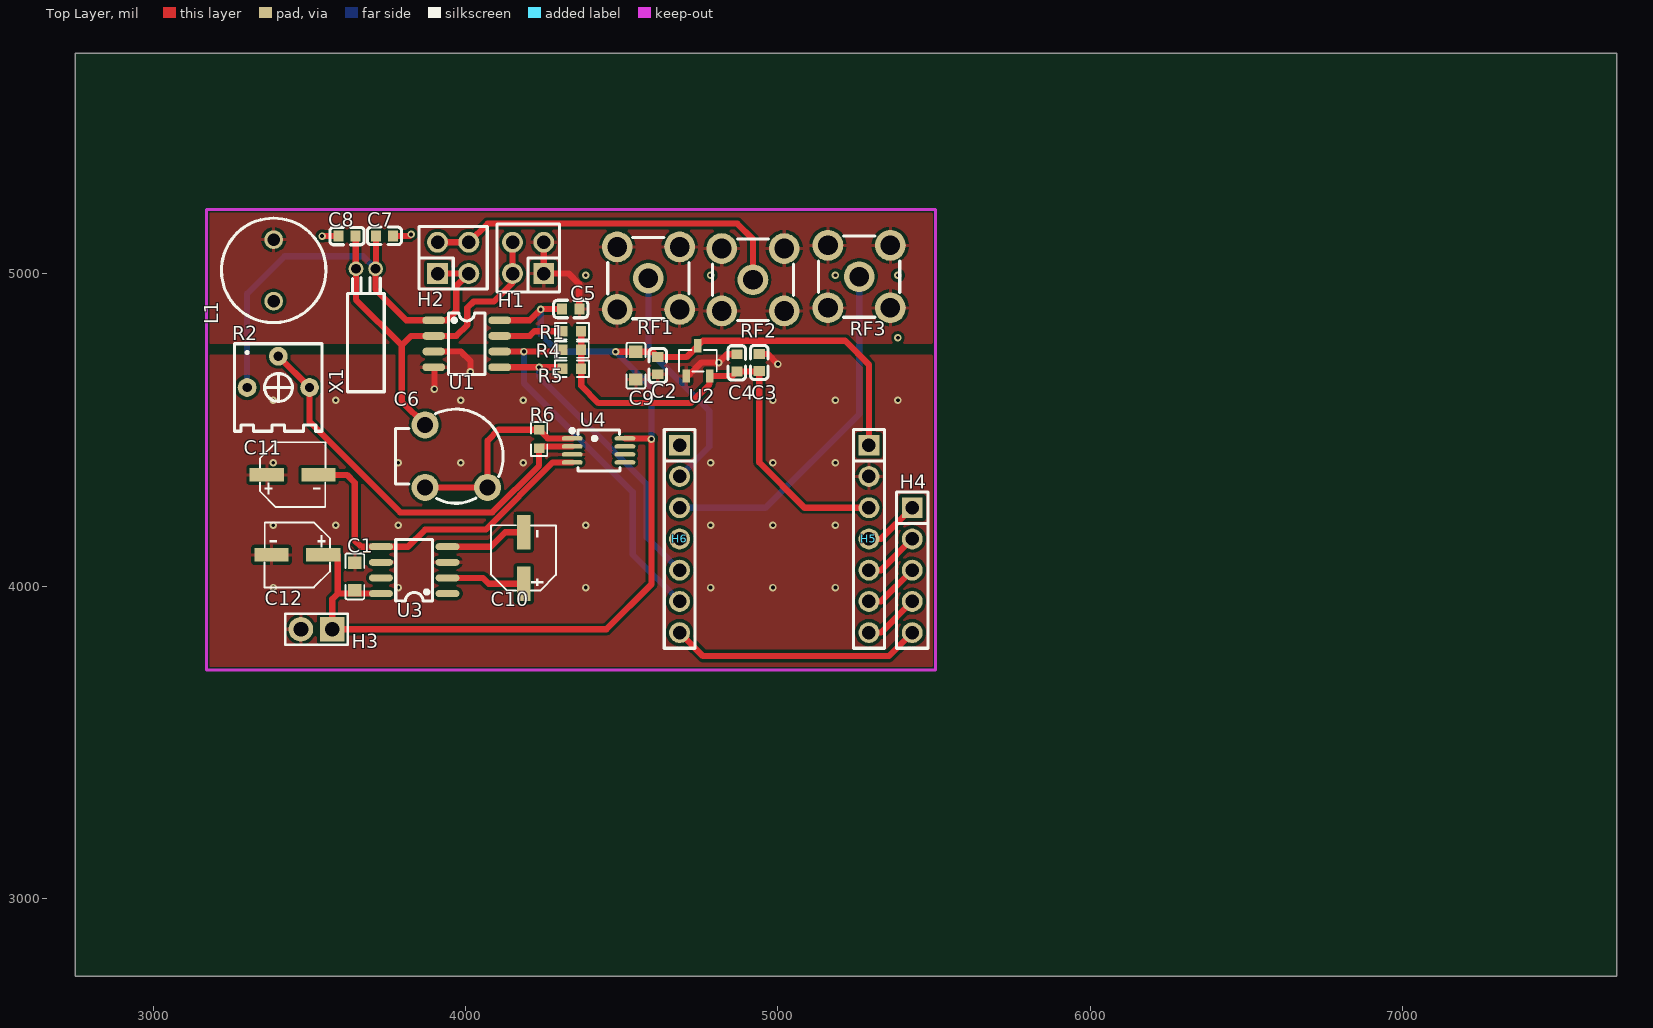
[diagram p0: Top Layer view]
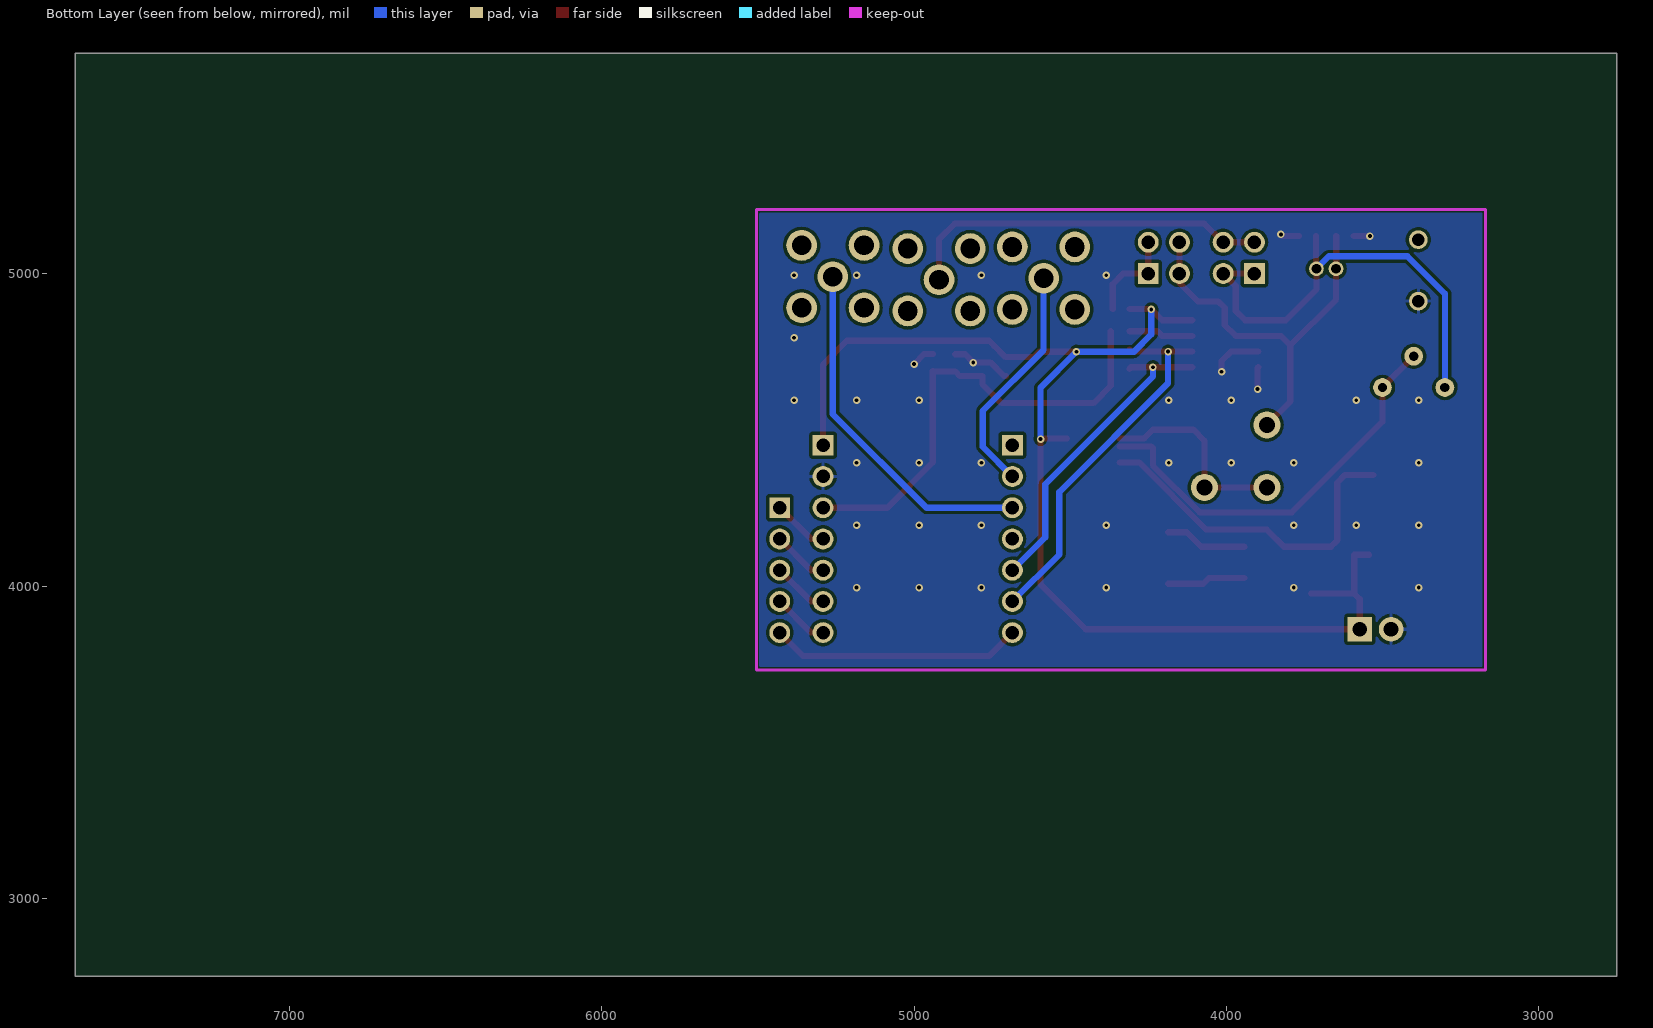
[diagram p1: Bottom Layer view, seen from below]
# Altium PCB MISC75269.pcbdoc
Units mil, origin at the board's own origin, x right, y up, seen from the top; angles counter-clockwise.
Board outline 4935.75 x 2955.94 mil, 2 copper layers (Top Layer, Bottom Layer), stack 62.206 mil thick; 32 components, 24 nets, 111 pads, 43 vias.

## Layer stack, top to bottom
Top Solder Mask Layer: solder mask 0.394, Dk 3.3
Top Layer: signal copper 1.379
Dielectric1: surface 59.449, FR4, Dk 4.5
Bottom Layer: signal copper 1.378
Bottom Solder Mask Layer: solder mask 0.394, Dk 3.3

## Board outline
7685.75,2750 2750,2750 2750,5705.94 7685.75,5705.94

## Design rules (kind name [scope] priority, off if disabled: settings)
BoardOutlineClearance copperThickness2oz_1 [All] p2 off: genericclearance=7.99 ignorepadtopadclearanceinfootprint=FALSE except(0: Arc-SplitContinuation Track-SplitContinuation SMDPad-SplitContinuation THPad-SplitContinuation Via-SplitContinuation Fill-SplitContinuation Region-SplitContinuation Poly-SplitContinuation Text-SplitContinuation Hole-SplitContinuation; 5.98: Arc-CutoutEdge SMDPad-CutoutEdge THPad-CutoutEdge Via-CutoutEdge Fill-CutoutEdge Region-CutoutEdge Text-CutoutEdge; 6.93: Hole-OutlineEdge Hole-CutoutEdge; 10: Poly-OutlineEdge Poly-CutoutEdge; 11.81: Arc-OutlineEdge Track-OutlineEdge SMDPad-OutlineEdge THPad-OutlineEdge Via-OutlineEdge Fill-OutlineEdge Region-OutlineEdge Text-OutlineEdge Track-CutoutEdge)
BoardOutlineClearance copperThickness1oz_1 [All] p4: genericclearance=4.02 ignorepadtopadclearanceinfootprint=FALSE except(0: Arc-SplitContinuation Track-SplitContinuation SMDPad-SplitContinuation THPad-SplitContinuation Via-SplitContinuation Fill-SplitContinuation Region-SplitContinuation Poly-SplitContinuation Text-SplitContinuation Hole-SplitContinuation; 6: SMDPad-CutoutEdge THPad-CutoutEdge Via-CutoutEdge Fill-CutoutEdge Region-CutoutEdge Text-CutoutEdge; 6.93: Hole-OutlineEdge Hole-CutoutEdge; 10: Poly-OutlineEdge Poly-CutoutEdge; 11.8: Arc-OutlineEdge Track-OutlineEdge SMDPad-OutlineEdge THPad-OutlineEdge Via-OutlineEdge Fill-OutlineEdge Region-OutlineEdge Text-OutlineEdge; 11.81: Arc-CutoutEdge Track-CutoutEdge)
Clearance copperThickness2oz [All] p1 off: gap=7.99 ignorepadtopadclearanceinfootprint=FALSE except(5.98: SMDPad-Track SMDPad-SMDPad THPad-Track SMDPad-THPad THPad-THPad Track-Via SMDPad-Via THPad-Via Via-Via Fill-Track Region-Track Fill-SMDPad Region-SMDPad Fill-THPad Region-THPad Fill-Via Region-Via Fill-Fill Fill-Region Region-Region Arc-Track Arc-SMDPad Arc-THPad Arc-Via Fill-Arc Region-Arc Arc-Arc Text-Track SMDPad-Text Text-THPad Text-Via Fill-Text Region-Text Arc-Text Text-Text; 6.93: Hole-Track Hole-SMDPad Hole-THPad Hole-Via Fill-Hole Region-Hole Hole-Arc Hole-Text; 10: Poly-Track Poly-SMDPad Poly-THPad Poly-Via Poly-Fill Poly-Region Poly-Poly Poly-Arc Poly-Text Poly-Hole)
Clearance copperThickness1oz [All] p3: gap=4.02 ignorepadtopadclearanceinfootprint=FALSE except(5.98: SMDPad-Track SMDPad-SMDPad THPad-Track SMDPad-THPad THPad-THPad Track-Via SMDPad-Via THPad-Via Via-Via Fill-Track Region-Track Fill-SMDPad Region-SMDPad Fill-THPad Region-THPad Fill-Via Region-Via Fill-Fill Fill-Region Region-Region; 6: Arc-Track Arc-SMDPad Arc-THPad Arc-Via Fill-Arc Region-Arc Arc-Arc Text-Track SMDPad-Text Text-THPad Text-Via Fill-Text Region-Text Arc-Text Text-Text; 6.93: Hole-Track Hole-SMDPad Hole-THPad Hole-Via Fill-Hole Region-Hole Hole-Arc Hole-Text; 10: Poly-Track Poly-SMDPad Poly-THPad Poly-Via Poly-Fill Poly-Region Poly-Poly Poly-Arc Poly-Text Poly-Hole)
DiffPairsRouting differentialPair [All] p1: maxlimit=6 minlimit=6 mostfreqgap=6 toplayer_minwidth=5 toplayer_prefwidth=10 toplayer_maxwidth=100 toplayer_mingap=6 toplayer_prefgap=6 toplayer_maxgap=6 bottomlayer_minwidth=5 bottomlayer_prefwidth=10 bottomlayer_maxwidth=100 bottomlayer_mingap=6 bottomlayer_prefgap=6 bottomlayer_maxgap=6 maxuncoupledlength=10
HoleToHoleClearance otherClearance [All] p1: gap=11.81 allowstackedmicrovias=TRUE
Length netLength [All] p1: minlimit=0 maxlimit=0
MatchedLengths netLengthTolerance [All] p1: tolerance=1000
PasteMaskExpansion pasteMaskExpansion [All] p1: expansion=0
PlaneConnect innerPlane [All] p1: planeconnectstyle=Relief reliefexpansion=20 reliefentries=4 reliefconductorwidth=10 reliefairgap=10
PolygonConnect copperRegion [(InNet('GND') OR InNet('PGND'))] p1: connectstyle=Relief reliefconductorwidth=10 reliefentries=4 polygonreliefangle="90 Angle" airgapwidth=10 via.connectstyle=Relief via.reliefconductorwidth=10 via.reliefentries=4 via.polygonreliefangle="90 Angle" via.airgapwidth=10
RoutingVias viaSize [All] p1: holewidth=12.01 width=24.02 viastyle="Through Hole" minholewidth=11.81 minwidth=19.68 maxholewidth=248.03 maxwidth=393.7
SolderMaskExpansion solderMaskExpansion [IsVia] p1: expansion=-1000 istentingtop=TRUE
SolderMaskExpansion solderMaskExpansion [All] p2: expansion=2 istentingtop=FALSE
Width copperThickness2oz_2 [All] p1 off: maxlimit=100 minlimit=8 preferedwidth=10
Width copperThickness1oz_2 [All] p2: maxlimit=100 minlimit=5 preferedwidth=10

## Components (designator, comment, footprint, x,y, rotation, side; value= is the part's Value field where it differs from the comment)
C1 "20uF" CAP-SMD_L1.8-W1.0 3645,4030.94 r270 top
C2 "100nF" C0603 4615,4705.94 r90 top
C3 "10uF" C0603 4940,4715.94 r270 top
C4 "100nF" C0603 4868.26,4715.05 r270 top
C5 "100nF" C0603 4336.39,4887.29 r180 top
C6 "3pF~33pF" CAP-ADJ-TH_3P-BD7.6_BFC280811339 3970,4415.94 r0 top
C7 "22pF" C0603 3739.97,5121.45 r0 top
C8 "22pF" C0603 3620,5120.94 r180 top
C9 "20uF" CAP-SMD_L1.8-W1.0 4545,4705.94 r90 top
C10 "10uF" CAP-SMD_BD5.0-L5.3-W5.3-LS6.0-FD 4185.76,4090.02 r90 top
C11 "10uF" CAP-SMD_BD5.0-L5.3-W5.3-LS6.0-FD 3446,4356.1 r0 top
C12 "10uF" CAP-SMD_BD5.0-L5.3-W5.3-LS6.0-FD 3460.76,4100.02 r180 top
H1 "PZ254V-12-4P" HDR-TH_4P-P2.54-V-M-R2-C2-S2.54 4200,5050.94 r90 top
H2 "PZ254V-12-4P" HDR-TH_4P-P2.54-V-M-R2-C2-S2.54 3960,5050.94 r0 top
H3 "PZ254V-11-02P" HDR-TH_2P-P2.54-V-M 3522.32,3861.57 r180 top
H4 "" HDR-TH_5P-P2.54-V-M 5430,4050.94 r270 top
H5 "PZ254V-11-07P" HDR-TH_7P-P2.54-V-M 5291.42,4150.94 r270 top
H6 "PZ254V-11-07P" HDR-TH_7P-P2.54-V-M 4685,4150.94 r270 top
L1 "1mH" IND-TH_BD8.5-P5.00-D0.6 3385,5010.94 r90 top
R1 "3.3kΩ" R0603 4340,4815.94 r0 top
R2 "20kΩ" RES-ADJ-TH_3362P 3400,4685.94 r0 top
R4 "3.3kΩ" R0603 4339.54,4757.38 r180 top
R5 "3.3kΩ" R0603 4340,4695.94 r180 top
R6 "10kΩ" R0603 4235,4470.94 r270 top
RF1 "-" SMA-TH_KH-SMA-KE-Z 4585.01,4985.94 r90 top
RF2 "-" SMA-TH_KH-SMA-KE-Z 4920,4980.94 r90 top
RF3 "-" SMA-TH_KH-SMA-KE-Z 5260.01,4990.94 r90 top
U1 "DS1307ZN+T&R" SOP-8_L4.9-W3.9-P1.27-LS6.0-BL 4003.35,4775.94 r270 top
U2 "ME6211A33M3G-N" SOT-23-3_L2.9-W1.6-P1.90-LS2.8-BR 4743.58,4721.17 r270 top
U3 "MAX660ESA+T" SOIC-8_L5.0-W4.0-P1.27-LS6.0-BL 3835.21,4051.1 r90 top
U4 "AD8512ARMZ-REEL" MSOP-8_L3.0-W3.0-P0.65-LS5.0-TL 4425.46,4434.35 r0 top
X1 "32.768kHz" OSC-TH_BD3.1-P0.8-D0.3 3680,5015.94 r90 top

## Footprints (in the part's own frame and the unit in brackets; to place one, negate y for a bottom-side part, rotate by r counter-clockwise, add the part's x,y. Pads: shape width x height; smd on the part's side, far side on the other; paste and mask are expansions set on the pad)
C0603 [mm]
  rect 0.8x0.9 smd: 1(-0.7,0) 2(0.7,0)
  silkscreen extent -1.39,-0.71 1.39,0.71
CAP-ADJ-TH_3P-BD7.6_BFC280811339 [mm]
  round 2.2 hole 1.3 paste+0 mask+0.05: 1(-2.54,2.54) 2(-2.54,-2.54) 3(2.54,-2.54)
  silkscreen extent -4.95,-3.83 3.81,3.83
CAP-SMD_BD5.0-L5.3-W5.3-LS6.0-FD [mm]
  rect 2.8x1.1 smd: 1(-2.1,0) 2(2.1,0)
  silkscreen extent -2.66,-2.62 2.66,2.65
CAP-SMD_L1.8-W1.0 [mm]
  rect 1.015x1.08 smd: 1(-1.128,0) 2(1.128,0)
  silkscreen extent -1.86,-0.77 1.86,0.77
HDR-TH_2P-P2.54-V-M [mm]
  rect 2x2 hole 1.2: 1(-1.27,0)
  round 2 hole 1.2: 2(1.27,0)
  silkscreen extent -2.54,-1.27 2.54,1.27
HDR-TH_4P-P2.54-V-M-R2-C2-S2.54 [mm]
  rect 1.7x1.7 hole 1.1: 1(-1.27,-1.27)
  round 1.7 hole 1.1: 2(-1.27,1.27) 3(1.27,-1.27) 4(1.27,1.27)
  silkscreen extent -2.77,-2.54 2.77,2.54
HDR-TH_5P-P2.54-V-M [mm]
  rect 1.7x1.7 hole 1.1: 1(-5.08,0)
  round 1.7 hole 1.1: 2(-2.54,0) 3(0,0) 4(2.54,0) 5(5.08,0)
  silkscreen extent -6.35,-1.27 6.35,1.27
HDR-TH_7P-P2.54-V-M [mm]
  rect 1.7x1.7 hole 1.1: 1(-7.62,0)
  round 1.7 hole 1.1: 2(-5.08,0) 3(-2.54,0) 4(0,0) 5(2.54,0) 6(5.08,0) 7(7.62,0)
  silkscreen extent -8.89,-1.25 8.89,1.25
IND-TH_BD8.5-P5.00-D0.6 [mil]
  round 60 hole 39.37: 1(-98.43,0) 2(98.42,0)
  silkscreen extent -167,-167 167,167
MSOP-8_L3.0-W3.0-P0.65-LS5.0-TL [mil]
  oval 66.61x14.33 smd: 1(-84.49,38.39) 2(-84.49,12.79) 3(-84.49,-12.8) 4(-84.49,-38.39) 5(84.49,-38.39) 6(84.49,-12.8) 7(84.49,12.79) 8(84.49,38.39)
  silkscreen extent -90,-65 68,69
OSC-TH_BD3.1-P0.8-D0.3 [mm]
  round 1.2 hole 0.8: 1(0,0.8) 2(0,-0.8)
  silkscreen extent -10,-1.5 -0.7,1.5
R0603 [mil]
  rect 31.75x34.02 smd paste-3937.01 mask+2: 1(-29.66,0) 2(29.66,0)
  silkscreen extent -55,-26 55,26
RES-ADJ-TH_3362P [mil]
  round 60 hole 30: 1(-100,-50) 2(0,50) 3(100,-50)
  silkscreen extent -140,-190 140,90
SMA-TH_KH-SMA-KE-Z [mm]
  round 2.5 hole 1.6 copper offset 0,0: 1(-2.54,-2.54) 2(-2.54,2.54) 3(2.54,2.54) 4(2.54,-2.54)
  round 2.5 hole 1.6: 5(0,0)
  silkscreen extent -3.3,-3.3 3.3,3.3
SOIC-8_L5.0-W4.0-P1.27-LS6.0-BL [mil]
  oval 22.38x76.78 smd: 1(-75,-106.5) 2(-25,-106.5) 3(25,-106.5) 4(75,-106.5) 5(75,106.5) 6(25,106.5) 7(-25,106.5) 8(-75,106.5)
  silkscreen extent -98,-59 98,59
SOP-8_L4.9-W3.9-P1.27-LS6.0-BL [mm]
  oval 0.63x1.865 smd: 1(-1.905,-2.682) 2(-0.635,-2.682) 3(0.635,-2.682) 4(1.905,-2.682) 5(1.905,2.682) 6(0.635,2.682) 7(-0.635,2.682) 8(-1.905,2.682)
  silkscreen extent -2.5,-1.5 2.5,1.48
SOT-23-3_L2.9-W1.6-P1.90-LS2.8-BR [mm]
  rect 1.07x0.6 smd: 1(1.235,-0.95) 2(1.235,0.95) 3(-1.235,0)
  silkscreen extent -0.88,-1.54 0.88,1.54

## Via types
v1: diameter 24.02, hole 12, Top Layer to Bottom Layer, 43 vias

## Nets (pads, with @x,y where several pads share a name; then routed paths per layer and width w, separated by ;. In a path a pad name is that pad's centre, name@x,y a point inside that pad or via, vN(x,y) a via of type N, cw(c..) or ccw(c..) an arc to the next point about the centre after c; other vN are vias at no path point)
3V3: C3.2 C4.2 H5.3 R1.2 R4.1 R5.1 U2.2 | length 1529.3
  Top Layer w20: R1.2 R5.1 4369.66,4641.28 4425,4585.94 4720,4585.94 4780.98,4646.92 U2.2 4853.32,4672.54 C4.2 4939.1,4687.49 C3.2 4940,4395.94 5085,4250.94 H5.3
$1N31: R1.1 U1.7 | length 207.6
  Top Layer w20: U1.7 4205,4800.94 4220,4815.94 R1.1
$1N157: C6.2 C6.3 R6.1 U4.1 | length 646.9
  Top Layer w20: C6.2 C6.3 4070,4465.94 4104.66,4500.6 R6.1 4262.87,4472.74 U4.1
$1N162: R2.2 R2.3 R6.2 U4.2 | length 1332.4
  Top Layer w20: R2.2 R2.3 3500,4525.94 3790,4235.94 4085,4235.94 4235,4385.94 R6.2 4240.85,4447.14 U4.2
$1N166: C10.1 U3.2 | length 251.8
  Top Layer w20: U3.2 4054.85,4026.1 4073.6,4007.35 C10.1
$1N167: C10.2 U3.4 | length 263.3
  Top Layer w20: U3.4 4080.15,4126.1 4126.75,4172.7 C10.2
$1N168: C11.2 U3.5 U4.4 | length 1127.7
  Top Layer w20: C11.2 3619.85,4356.1 3645,4330.94 3645,4145.94 3664.85,4126.1 U3.5 3815.15,4126.1 3870,4180.94 4063.96,4180.94 4278.98,4395.96 U4.4
A: C7.1 H2.1 H2.3 R2.1 U1.1 X1.2 | length 1498.5
  Top Layer w20: C7.1 3712.41,5016.85 X1.2 3711.5,4949.44 3810,4850.94 U1.1 3940,4850.94 3970,4880.94 3970,4960.94 H2.3 H2.1
  Bottom Layer w20: R2.1 3300,4935.94 3420,5055.94 3671.5,5055.94 X1.2
B: C6.1 C8.1 H1.2 H1.4 U1.2 X1.1 | length 1297.2
  Top Layer w20: C8.1 3647.56,5016.89 X1.1 3648.5,4917.44 3795,4770.94 ; C6.1 3795,4590.94 3795,4770.94 ; H1.4 H1.2 4150,4970.94 4090,4910.94 4025,4910.94 4005,4890.94 4005,4835.94 3970,4800.94 U1.2 3825,4800.94 3795,4770.94
D0: H6.1
D1: H6.2 RF1.5 | length 755.1
  Bottom Layer w20: RF1.5 4585,4755.95 4780,4560.94 4780,4445.94 H6.2
D2: H6.3 RF3.5 | length 1139.2
  Bottom Layer w20: H6.3 4960,4250.94 5260,4550.94 RF3.5
D3: H6.4
D4: H6.5 R5.2 U1.5 | length 1039.8
  Top Layer w20: U1.5 v1(4235.02,4700.94) 4305.34,4700.94 R5.2
  Bottom Layer w20: v1(4235.02,4700.94) 4235.02,4670.93 4580,4325.94 4580,4155.94 H6.5
D5: H6.6 R4.2 U1.6 | length 1210
  Top Layer w20: U1.6 v1(4186.65,4750.94) 4303.44,4750.94 R4.2
  Bottom Layer w20: v1(4186.65,4750.94) 4186.65,4649.3 4535,4300.94 4535,4100.94 H6.6
D6: H4.5 H6.7 | length 807.1
  Top Layer w20: H6.7 4760,3775.94 5355,3775.94 H4.5
D7: H4.4 H5.7 | length 180
  Top Layer w20: H5.7 5330,3850.94 H4.4
D8: H4.3 H5.6 | length 180
  Top Layer w20: H5.6 5330,3950.94 H4.3
D9: H4.2 H5.5 | length 180
  Top Layer w20: H5.5 5330,4050.94 H4.2
D10: H4.1 H5.4 | length 180
  Top Layer w20: H5.4 5330,4150.94 H4.1
GND: C1.1 C2.1 C3.1 C4.1 C7.2 C8.2 C9.1 C11.1 C12.2 H3.2 H5.2 L1.1 U1.3 U1.4 U2.1 U3.3 U3.6 U4.3 | length 612
  Top Layer w20: v1(3540,5120.94) C8.2 ; C7.2 3820.51,5121.45 v1(3825,5125.94) ; U1.4 3900,4698.69 v1(3900,4630.94) ; U1.3 3985,4750.94 4015,4720.94 v1(4015,4685.94) ; U2.1 4711.6,4672.54 4755,4715.94 v1(4810,4715.94) 4836.66,4742.61 C4.1 ; C3.1 4967.44,4743.5 v1(5000,4710.94)
  other v1: 3384.1,3995.04 3784.1,3995.04 4384.1,3995.04 4784.1,3995.04 4984.1,3995.04 5184.1,3995.04 3384.1,4195.04 3584.1,4195.04 3784.1,4195.04 4384.1,4195.04 4784.1,4195.04 4984.1,4195.04 5184.1,4195.04 3384.1,4395.04 3784.1,4395.04 3984.1,4395.04 4184.1,4395.04 4784.1,4395.04 4984.1,4395.04 5184.1,4395.04 3384.1,4595.04 3584.1,4595.04 3984.1,4595.04 4184.1,4595.04 4984.1,4595.04 5184.1,4595.04 5384.1,4595.04 5384.1,4795.04 4384.1,4995.04 4784.1,4995.04 5184.1,4995.04 5384.1,4995.04
PGND: C5.1 H1.1 H1.3 L1.2 RF1.1 RF1.2 RF1.3 RF1.4 RF2.1 RF2.2 RF2.3 RF2.4 RF3.1 RF3.2 RF3.3 RF3.4 | length 307.7
  Top Layer w20: H1.3 H1.1 4330,5000.94 4363.95,4966.99 C5.1
TIP: H2.2 H2.4 RF2.5 | length 1185.6
  Top Layer w20: H2.2 H2.4 4070,5160.94 4870,5160.94 4919.99,5110.95 RF2.5
VCC: C1.2 C2.2 C5.2 C9.2 C12.1 H3.1 H5.1 U1.8 U2.3 U3.8 U4.8 | length 4076.8
  Top Layer w20: C12.1 3590.15,4100.02 3590.15,3976.1 ; U3.8 3590.15,3976.1 ; U1.8 4205,4850.94 4241.34,4887.29 C5.2 ; v1(4480,4750.33) C9.2 4598.17,4750.33 C2.2 4707.29,4733.5 U2.3 4759.73,4785.94 5215,4785.94 5291.42,4709.52 H5.1 ; U4.8 4588.21,4472.74 4595,4465.94 4595,4005.94 4450.63,3861.57 H3.1 3572.32,3958.26 3590.15,3976.1
  Bottom Layer w20: v1(4240,4885.94) 4240,4805.94 4295.61,4750.33 v1(4480,4750.33) 4595,4635.33 v1(4595,4470.94)
pads on no net: U3.1 U3.7 U4.5 U4.6 U4.7

## Polygon pours and split planes (outlines as drawn)
GND on Top Layer (solid, remove dead copper, pour order 0): 3000,4740.94 3000,3620.94 5555,3620.94 5555,4740.94
GND on Bottom Layer (solid, remove dead copper, pour order 4): 3055,5345.94 3055,3640.94 5560,3640.94 5560,5345.94
PGND on Top Layer (solid, remove dead copper, pour order 2): 3095,5455.94 3095,4775.94 5620,4775.94 5620,5455.94

## Keep-outs
Board Outline Layer:
  lines w10: 3170,3730.94 3170,5205.94 5505,5205.94 5505,3730.94 3170,3730.94